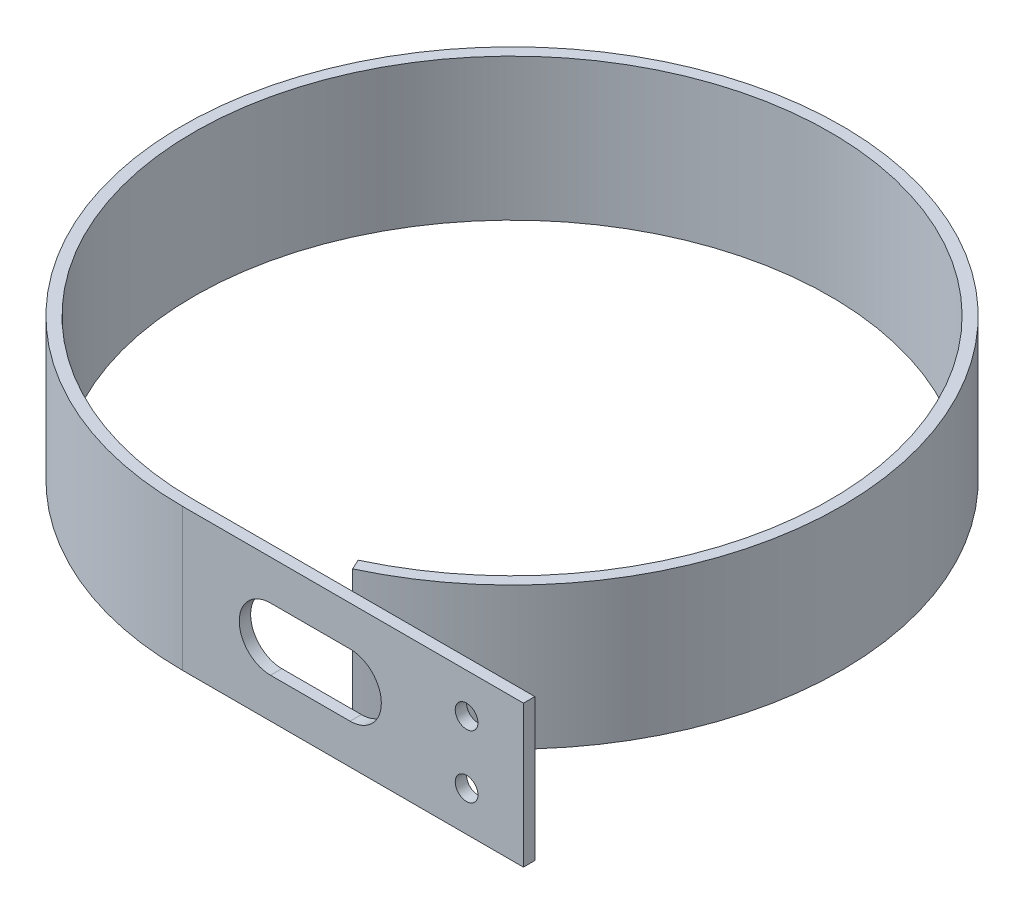
SolidWorks part; units mm, degrees
material "A3"
ref_plane "前视基准面" through (0, 0, 0) normal (0, 0, 1) x (1, 0, 0)
ref_plane "上视基准面" through (0, 0, 0) normal (0, 1, 0) x (1, 0, 0)
ref_plane "右视基准面" through (0, 0, 0) normal (1, 0, 0) x (0, 0, -1)
sketch "草图1" plane through (0, 0, 0) normal (0, 1, 0) x (1, 0, 0)
  line L0 (0, -56) -> (60, -56)
  line L1 (0, 0) -> (30.5595, -65.5352) construction
  line L2 (0, 0) -> (0, -56) construction
  arc A0 (23.6666, -50.7532) -> (0, -56) centre (0, 0) ccw
  dimension "D1" = 112
  dimension "D2" = 60
  dimension "D3" = 25
extrude "拉伸-薄壁1" add sketch "草图1" along normal mid plane 25 thin
sketch "草图3" plane through (0, 0, 58) normal (0, 0, 1) x (1, 0, 0)
  line L0 (15.5, 0) -> (29.5, 0) construction
  line L1 (15.5, 5.5) -> (29.5, 5.5)
  line L2 (15.5, -5.5) -> (29.5, -5.5)
  line L3 (60, 12.5) -> (60, -12.5) construction
  line L4 (0, 0) -> (10, 0) construction
  arc A0 (15.5, 5.5) -> (15.5, -5.5) centre (15.5, 0) ccw
  arc A1 (29.5, -5.5) -> (29.5, 5.5) centre (29.5, 0) ccw
  circle A2 centre (50, 5.5) radius 2
  circle A3 centre (50, -5.5) radius 2
  point P3 (22.5, 0)
  point P8 (10, 0)
  point P9 (35, 0)
  dimension "D4" = 4
  dimension "D1" = 11
  dimension "D2" = 25
  dimension "D3" = 25
  dimension "D5" = 10
extrude "切除-拉伸1" cut sketch "草图3" against normal blind 2
